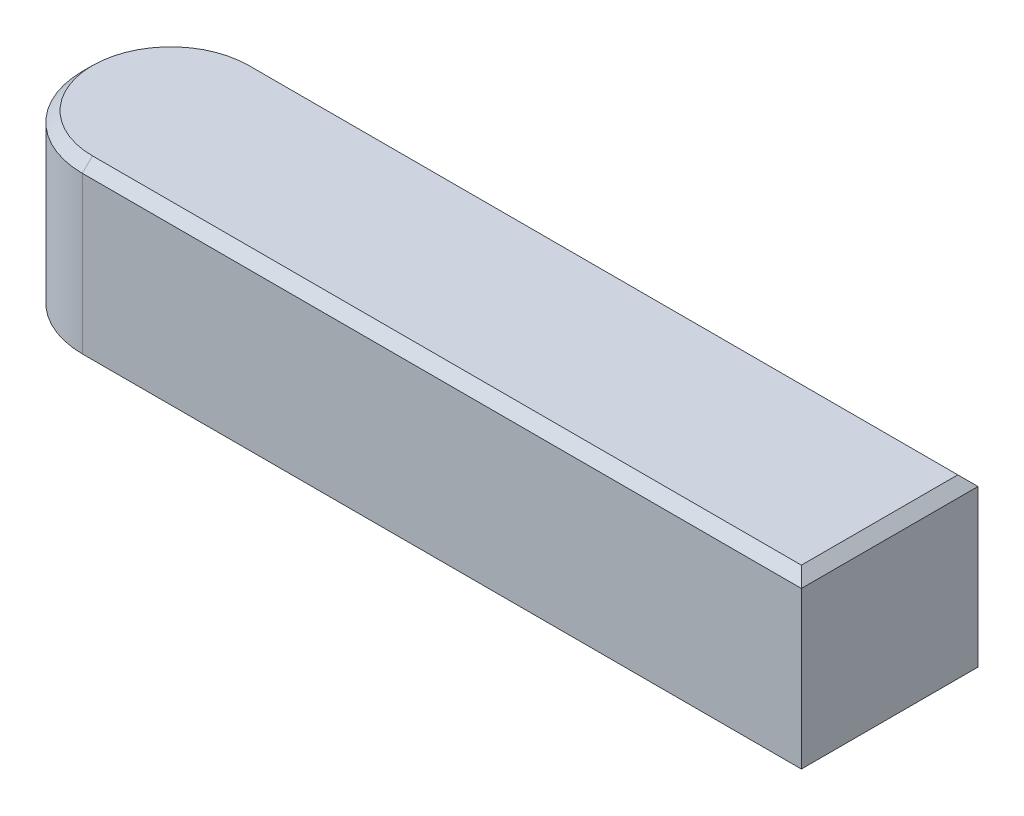
from build123d import *

# Parameters (mm, degrees)
EXTRUDE_1_DEPTH = 7
CHAMFER_1_SIZE  = 0.4


with BuildPart() as part:
    # 草图1 → 凸台-拉伸1 (new body)
    with BuildSketch(Plane(origin=(0, 0, 0), x_dir=(1, 0, 0), z_dir=(0, 1, 0))):
        with BuildLine():
            Line((3.5, 0), (32, 0))
            Line((32, 0), (32, -7))
            Line((32, -7), (3.5, -7))
            ThreePointArc((3.5, -7), (0, -3.5), (3.5, 0))
        make_face()
    extrude(amount=EXTRUDE_1_DEPTH)

    # 倒角1
    chamfer_1_edges = [part.edges().sort_by_distance(p)[0] for p in [
        (32, 7, 3.5),
        (17.75, 7, 0),
        (0, 7, 3.5),
        (17.75, 0, 0),
        (32, 0, 3.5),
        (17.75, 0, 7),
        (0, 0, 3.5),
        (17.75, 7, 7),
    ]]
    chamfer(chamfer_1_edges, length=CHAMFER_1_SIZE)


solid = part.part
